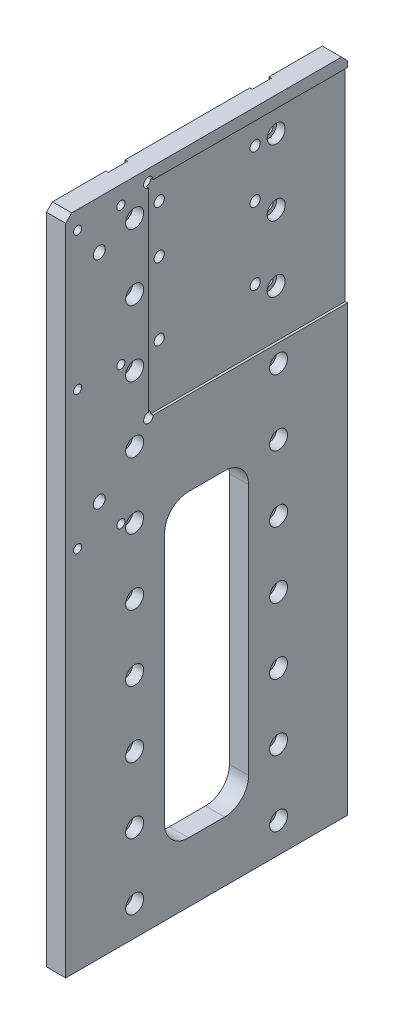
SolidWorks part; units mm, degrees
material "6061-T4 (SS)"
ref_plane "前视基准面" through (0, 0, 0) normal (0, 0, 1) x (1, 0, 0)
ref_plane "上视基准面" through (0, 0, 0) normal (0, 1, 0) x (1, 0, 0)
ref_plane "右视基准面" through (0, 0, 0) normal (1, 0, 0) x (0, 0, -1)
sketch "草图1" plane through (0, 0, 0) normal (0, 0, 1) x (1, 0, 0)
  line L1 (-8, -275) -> (8, -275)
  line L2 (-8, -275) -> (-8, 275)
  line L3 (-8, 275) -> (8, 275)
  line L4 (8, -275) -> (8, 275)
  line L5 (0, 275) -> (0, -275) construction
  line L6 (-8, 0) -> (8, 0) construction
  point P0 (0, 0)
  dimension "D1" = 16
  dimension "D2" = 550
extrude "凸台-拉伸1" add sketch "草图1" along normal blind 235
sketch "草图4" plane through (-8, 0, 0) normal (-1, 0, 0) x (0, 0, 1)
  line L0 (117.5, 275) -> (117.5, -275) construction
  line L3 (235, 275) -> (0, 275) construction
  line L4 (235, -275) -> (0, -275) construction
  line L5 (57.5, 275) -> (57.5, -275) construction
  line L6 (177.5, 275) -> (177.5, -275) construction
  line L8 (49.5, -275) -> (65.5, -275)
  line L9 (49.5, -275) -> (49.5, 275)
  line L10 (49.5, 275) -> (65.5, 275)
  line L11 (65.5, -275) -> (65.5, 275)
  line L12 (57.5, 275) -> (57.5, -275) construction
  line L13 (49.5, 0) -> (65.5, 0) construction
  line L14 (169.5, -275) -> (185.5, -275)
  line L15 (169.5, -275) -> (169.5, 275)
  line L16 (169.5, 275) -> (185.5, 275)
  line L17 (185.5, -275) -> (185.5, 275)
  line L18 (177.5, 275) -> (177.5, -275) construction
  line L19 (169.5, 0) -> (185.5, 0) construction
  point P10 (177.5, 0)
  point P11 (57.5, 0)
  dimension "D1" = 120
  dimension "D2" = 16
extrude "切除-拉伸3" cut sketch "草图4" against normal blind 2
sketch "草图5" plane through (8, 0, 0) normal (1, 0, 0) x (0, 0, -1)
  line L0 (0, -275) -> (0, 275) construction
  line L1 (-166, 265) -> (0, 265)
  line L2 (-166, 265) -> (-166, 95)
  line L3 (-166, 95) -> (0, 95)
  line L4 (0, 265) -> (0, 95)
  line L7 (-235, 275) -> (0, 275) construction
  dimension "D1" = 10
  dimension "D2" = 170
  dimension "D3" = 166
extrude "切除-拉伸4" cut sketch "草图5" against normal blind 2
hole_wizard "M10 螺纹孔1" positions "草图6" profile "草图7" tap size "M10" standard "GB"
sketch "草图6" plane through (6, 0, 0) normal (1, 0, 0) x (0, 0, -1)
  line L11 (-155, 245) -> (-75, 245) construction
  line L12 (-155, 245) -> (-155, 145) construction
  line L13 (-155, 145) -> (-75, 145) construction
  line L14 (-75, 245) -> (-75, 145) construction
  line L15 (0, 265) -> (-166, 265) construction
  line L19 (-235, 265) -> (-235, 95) construction
  line L20 (-75, 205) -> (-155, 205) construction
  point P156 (-155, 245)
  point P157 (-75, 145)
  point P226 (-155, 145)
  point P227 (-75, 245)
  point P236 (-75, 205)
  point P242 (-155, 205)
  dimension "D1" = 80
  dimension "D2" = 100
  dimension "D3" = 20
  dimension "D4" = 60
  dimension "D6" = 80
sketch "草图7" plane through (6, 245, 155) normal (0, 1, 0) x (0, 0, -1)
  line L0 (0, 0) -> (0, 30.0537)
  line L1 (0, 30.0537) -> (4.25, 27.5)
  line L2 (4.25, 27.5) -> (4.25, 0)
  line L5 (4.25, 0) -> (0, 0)
  line L10 (0, 30.0537) -> (-4.25, 27.5) construction
  line L11 (0, -6.35) -> (0, 107.95) construction
  dimension "螺纹孔钻头直径" = 8.5
  dimension "螺纹孔钻头深度" = 27.5
  dimension "导头角度" = 118
cosmetic thread "孔螺蚊线20" parameters "D1"=14, "D2"=10
cosmetic thread "孔螺蚊线21" parameters "D1"=14, "D2"=10
cosmetic thread "孔螺蚊线22" parameters "D1"=14, "D2"=10
cosmetic thread "孔螺蚊线23" parameters "D1"=14, "D2"=10
cosmetic thread "孔螺蚊线24" parameters "D1"=14, "D2"=10
cosmetic thread "孔螺蚊线25" parameters "D1"=14, "D2"=10
hole_wizard "M8 螺纹孔1" positions "草图8" profile "草图9" tap size "M8" standard "GB"
sketch "草图8" plane through (0, -275, 0) normal (0, -1, 0) x (-1, 0, 0)
  line L0 (0, 0) -> (0, -235) construction
  line L1 (8, -235) -> (-8, -235) construction
  point P9 (0, -72.5)
  point P11 (0, -27.5)
  point P33 (0, -117.5)
  point P35 (0, -162.5)
  point P37 (0, -207.5)
  dimension "D1" = 27.5
  dimension "D2" = 45
  dimension "D3" = 45
  dimension "D4" = 45
  dimension "D5" = 45
sketch "草图9" plane through (0, -275, 207.5) normal (1, 0, 0) x (0, 0, -1)
  line L0 (0, 0) -> (0, 24.2929)
  line L1 (0, 24.2929) -> (3.4, 22.25)
  line L2 (3.4, 22.25) -> (3.4, 0)
  line L5 (3.4, 0) -> (0, 0)
  line L10 (0, 24.2929) -> (-3.4, 22.25) construction
  line L11 (0, -6.35) -> (0, 107.95) construction
  dimension "螺纹孔钻头直径" = 6.8
  dimension "螺纹孔钻头深度" = 22.25
  dimension "导头角度" = 118
cosmetic thread "孔螺蚊线7" parameters "D1"=16, "D2"=8
cosmetic thread "孔螺蚊线8" parameters "D1"=16, "D2"=8
cosmetic thread "孔螺蚊线9" parameters "D1"=16, "D2"=8
cosmetic thread "孔螺蚊线10" parameters "D1"=16, "D2"=8
cosmetic thread "孔螺蚊线11" parameters "D1"=16, "D2"=8
sketch "草图15" plane through (-8, 0, 0) normal (-1, 0, 0) x (0, 0, 1)
  line L0 (117.5, 275) -> (117.5, -275) construction
  line L1 (169.5, 275) -> (65.5, 275) construction
  line L2 (169.5, -275) -> (65.5, -275) construction
  line L4 (82.5, -225) -> (152.5, -225)
  line L5 (82.5, -225) -> (82.5, 25)
  line L6 (82.5, 25) -> (152.5, 25)
  line L7 (152.5, -225) -> (152.5, 25)
  line L8 (117.5, 25) -> (117.5, -225) construction
  line L9 (82.5, -100) -> (152.5, -100) construction
  point P6 (117.5, -100)
  dimension "D1" = 70
  dimension "D2" = 250
  dimension "D3" = 250
extrude "切除-拉伸5" cut sketch "草图15" against normal blind 16
fillet "圆角1" radius 20 4 edges at (0, -225, 82.5) (0, -225, 152.5) (0, 25, 152.5) (0, 25, 82.5)
chamfer "倒角1" distance 5 angle 45 2 edges at (0, 275, 0) (0, 275, 235)
hole_wizard "打孔尺寸(%根据)内六角圆柱头螺钉的类型1" positions "草图16" profile "草图17" counterbore size "M8" standard "GB"
sketch "草图16" plane through (8, 0, 0) normal (1, 0, 0) x (0, 0, -1)
  line L0 (-117.5, 275) -> (-117.5, -275) construction
  line L1 (-230, 275) -> (-5, 275) construction
  line L2 (-235, -275) -> (0, -275) construction
  line L3 (-177.5, -307.5) -> (-177.5, 275) construction
  line L4 (-57.5, -307.5) -> (-57.5, 275) construction
  line L5 (-177.5, -250) -> (-57.5, -250) construction
  point P15 (-177.5, -250)
  point P19 (-57.5, -250)
  dimension "D1" = 120
  dimension "D2" = 25
sketch "草图17" plane through (8, -250, 57.5) normal (0, 1, 0) x (0, 0, -1)
  line L0 (0, 0) -> (0, 30.2039)
  line L1 (0, 30.2039) -> (4.5, 27.5)
  line L2 (4.5, 27.5) -> (4.5, 9)
  line L3 (4.5, 9) -> (7.5, 9)
  line L4 (7.5, 9) -> (7.5, 0)
  line L5 (7.5, 0) -> (0, 0)
  line L10 (0, 30.2039) -> (-4.5, 27.5) construction
  line L11 (0, -6.35) -> (0, 107.95) construction
  dimension "孔直径" = 9
  dimension "孔深度" = 27.5
  dimension "柱形沉头孔直径" = 15
  dimension "柱形沉头孔深度" = 9
  dimension "导头角度" = 118
pattern_linear "阵列(线性)1" count 10 spacing 55 along (0, 1, 0) of "打孔尺寸(%根据)内六角圆柱头螺钉的类型1"
hole_wizard "M8 螺纹孔2" positions "草图18" profile "草图19" tap size "M8" standard "GB"
sketch "草图18" plane through (8, 0, 0) normal (1, 0, 0) x (0, 0, -1)
  line L2 (-189, 260) -> (-189, 28.6028) construction
  line L4 (-225, 260) -> (-225, 30) construction
  line L5 (-207, 30) -> (-207, 260) construction
  line L6 (-189, 145) -> (-225, 145) construction
  line L9 (-189, 30) -> (-225, 30) construction
  line L11 (-189, 260) -> (-225, 260) construction
  line L12 (-230, 275) -> (-5, 275) construction
  line L13 (-235, -275) -> (-235, 270) construction
  point P312 (-189, 145)
  point P314 (-225, 145)
  point P323 (-189, 260)
  point P325 (-225, 260)
  point P327 (-189, 30)
  point P329 (-225, 30)
  dimension "D1" = 36
  dimension "D2" = 15
  dimension "D3" = 10
  dimension "D6" = 230
sketch "草图19" plane through (8, 30, 225) normal (0, 1, 0) x (0, 0, -1)
  line L0 (0, 0) -> (0, 24.2929)
  line L1 (0, 24.2929) -> (3.4, 22.25)
  line L2 (3.4, 22.25) -> (3.4, 0)
  line L5 (3.4, 0) -> (0, 0)
  line L10 (0, 24.2929) -> (-3.4, 22.25) construction
  line L11 (0, -6.35) -> (0, 107.95) construction
  dimension "螺纹孔钻头直径" = 6.8
  dimension "螺纹孔钻头深度" = 22.25
  dimension "导头角度" = 118
cosmetic thread "孔螺蚊线12" parameters "D1"=16, "D2"=8
cosmetic thread "孔螺蚊线13" parameters "D1"=16, "D2"=8
cosmetic thread "孔螺蚊线14" parameters "D1"=16, "D2"=8
cosmetic thread "孔螺蚊线15" parameters "D1"=16, "D2"=8
cosmetic thread "孔螺蚊线26" parameters "D1"=16, "D2"=8
cosmetic thread "孔螺蚊线27" parameters "D1"=16, "D2"=8
sketch "草图20" plane through (8, 0, 0) normal (1, 0, 0) x (0, 0, -1)
  circle A0 centre (-166, 95) radius 4
  circle A1 centre (-166, 265) radius 4
  dimension "D1" = 8
extrude "切除-拉伸6" cut sketch "草图20" against normal through all
hole_wizard "大小mm 暗销孔1" positions "草图21" profile "草图22" hole size "Ø10.0" standard "GB"
sketch "草图21" plane through (8, 0, 0) normal (1, 0, 0) x (0, 0, -1)
  line L0 (-189, 30) -> (-225, 30) construction
  line L1 (-207, 30) -> (-207, 262.8572) construction
  point P8 (-207, 55)
  point P10 (-207, 235)
  dimension "D1" = 25
  dimension "D2" = 180
sketch "草图22" plane through (8, 235, 207) normal (0, 1, 0) x (0, 0, -1)
  line L0 (0, 0) -> (0, 13.0043)
  line L1 (0, 13.0043) -> (5, 10)
  line L2 (5, 10) -> (5, 0)
  line L5 (5, 0) -> (0, 0)
  line L10 (0, 13.0043) -> (-5, 10) construction
  line L11 (0, -6.35) -> (0, 107.95) construction
  dimension "孔直径" = 10
  dimension "孔深度" = 10
  dimension "导头角度" = 118
